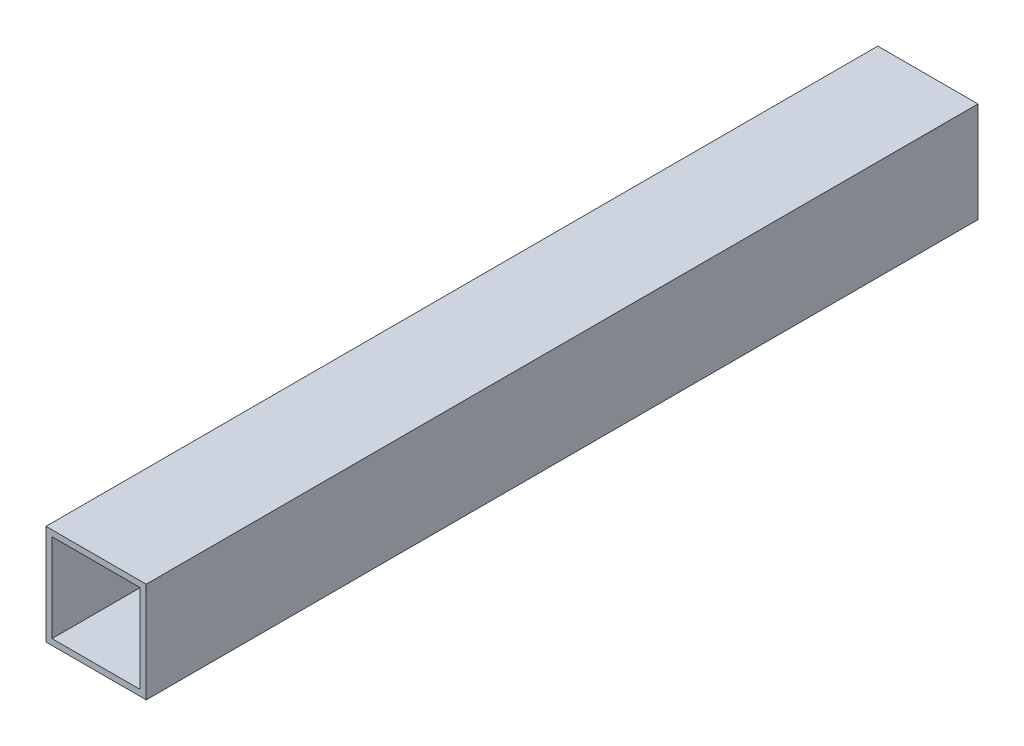
from build123d import *

# Parameters (mm, degrees)
SKETCH_1_W      = 50
SKETCH_1_H      = 50
SKETCH_1_W_2    = 44
SKETCH_1_H_2    = 44
EXTRUDE_1_DEPTH = 415


with BuildPart() as part:
    # 草图1 → 凸台-拉伸1 (new body)
    with BuildSketch(Plane.XY):
        with Locations((25, 25)):
            Rectangle(SKETCH_1_W, SKETCH_1_H)
        with Locations((25, 25)):
            Rectangle(SKETCH_1_W_2, SKETCH_1_H_2, mode=Mode.SUBTRACT)
    extrude(amount=EXTRUDE_1_DEPTH)


solid = part.part
